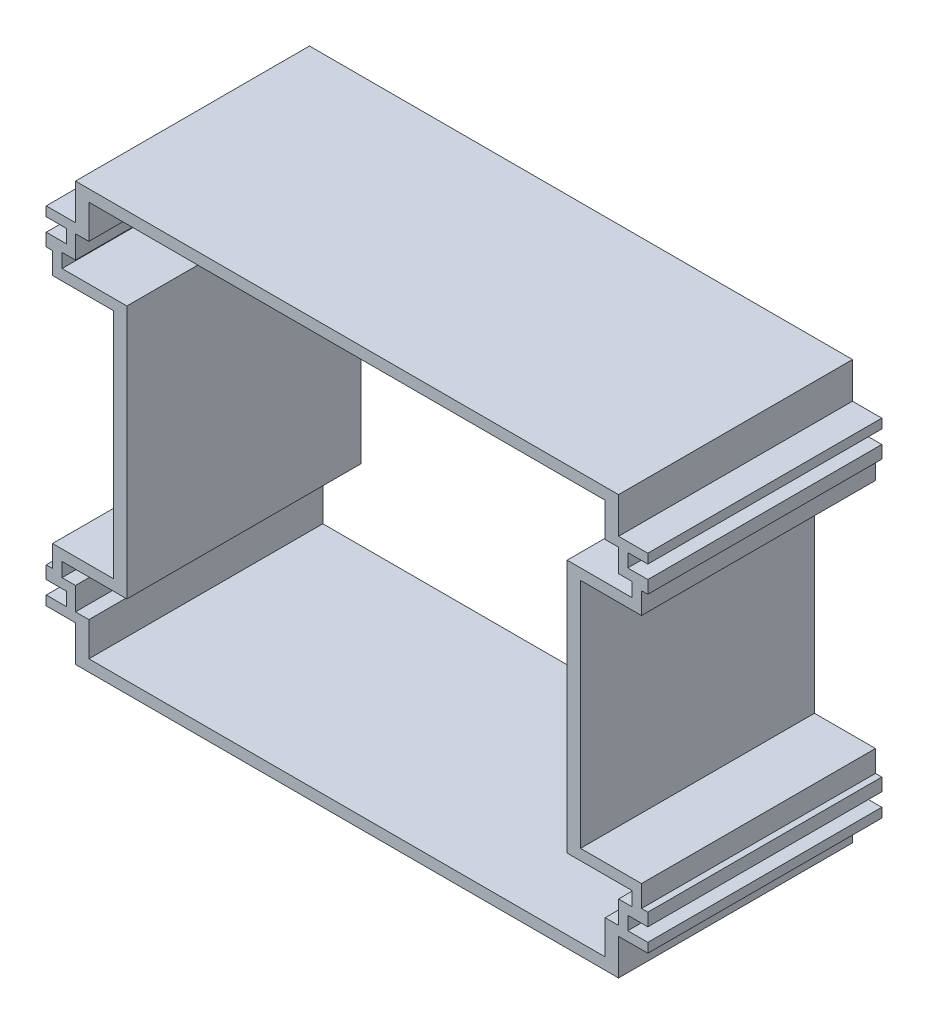
from build123d import *

# Parameters (mm, degrees)
BOSS_EXTRUDE1_START = -70
BOSS_EXTRUDE1_DEPTH = 70


with BuildPart() as part:
    # Sketch1 → Boss-Extrude1 (new body)
    with BuildSketch(Plane.XY.offset(BOSS_EXTRUDE1_START)):
        Polygon((90, 49), (84, 49), (84, 45), (90, 45), (90, 41.181900725), (88.106898586, 41.181900725), (88.106898586, 34.71973643), (69.860787635, 34.71973643), (69.860787635, -34.71973643), (88.106898586, -34.71973643), (88.106898586, -41.181900725), (90, -41.181900725), (90, -45), (84, -45), (84, -49), (90, -49), (90, -51.82740617), (81.240122505, -51.82740617), (81.240122505, -62.626229996), (-81.240122505, -62.626229996), (-81.240122505, -51.82740617), (-90, -51.82740617), (-90, -49), (-84, -49), (-84, -45), (-90, -45), (-90, -41.181900725), (-88.106898586, -41.181900725), (-88.106898586, -34.71973643), (-69.860787635, -34.71973643), (-69.860787635, 34.71973643), (-88.106898586, 34.71973643), (-88.106898586, 41.181900725), (-90, 41.181900725), (-90, 45), (-84, 45), (-84, 49), (-90, 49), (-90, 51.82740617), (-81.240122505, 51.82740617), (-81.240122505, 62.626229996), (81.240122505, 62.626229996), (81.240122505, 51.82740617), (90, 51.82740617), align=None)
        Polygon((65.860787635, -37.950818577), (65.860787635, 37.950818577), (85.261500452, 37.950818577), (85.261500452, 42.147480982), (81.240122505, 42.147480982), (81.240122505, 49), (77.240122505, 49), (77.240122505, 59.163837684), (-77.240122505, 59.163837684), (-77.240122505, 49), (-81.240122505, 49), (-81.240122505, 42.147480982), (-85.261500452, 42.147480982), (-85.261500452, 37.950818577), (-65.860787635, 37.950818577), (-65.860787635, -37.950818577), (-85.261500452, -37.950818577), (-85.261500452, -42.147480982), (-81.240122505, -42.147480982), (-81.240122505, -49), (-77.240122505, -49), (-77.240122505, -59.163837684), (77.240122505, -59.163837684), (77.240122505, -49), (81.240122505, -49), (81.240122505, -42.147480982), (85.261500452, -42.147480982), (85.261500452, -37.950818577), align=None, mode=Mode.SUBTRACT)
    extrude(amount=BOSS_EXTRUDE1_DEPTH)


solid = part.part
